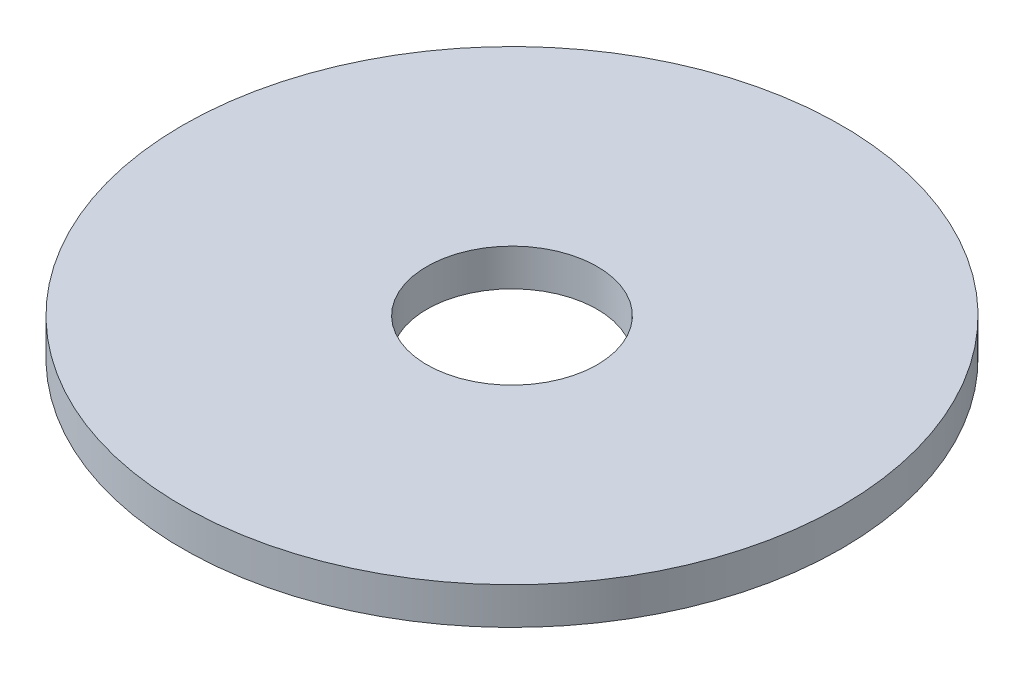
SolidWorks part; units mm, degrees
material "Plain Carbon Steel"
ref_plane "Front Plane" through (0, 0, 0) normal (0, 0, 1) x (1, 0, 0)
ref_plane "Top Plane" through (0, 0, 0) normal (0, 1, 0) x (1, 0, 0)
ref_plane "Right Plane" through (0, 0, 0) normal (1, 0, 0) x (0, 0, -1)
sketch "Sketch1" plane through (0, 0, 0) normal (0, 0, 1) x (1, 0, 0)
  line L0 (0, -799.8688) -> (0, 39193.5696) construction
  line L2 (11.5, 0) -> (44.5, 0)
  line L3 (11.5, 0) -> (11.5, 5)
  line L4 (11.5, 5) -> (44.5, 5)
  line L5 (44.5, 0) -> (44.5, 5)
  dimension "D1" = 11.5
  dimension "D2" = 44.5
  dimension "D3" = 5
revolve "Revolve1" add sketch "Sketch1" angle 360 about L0
